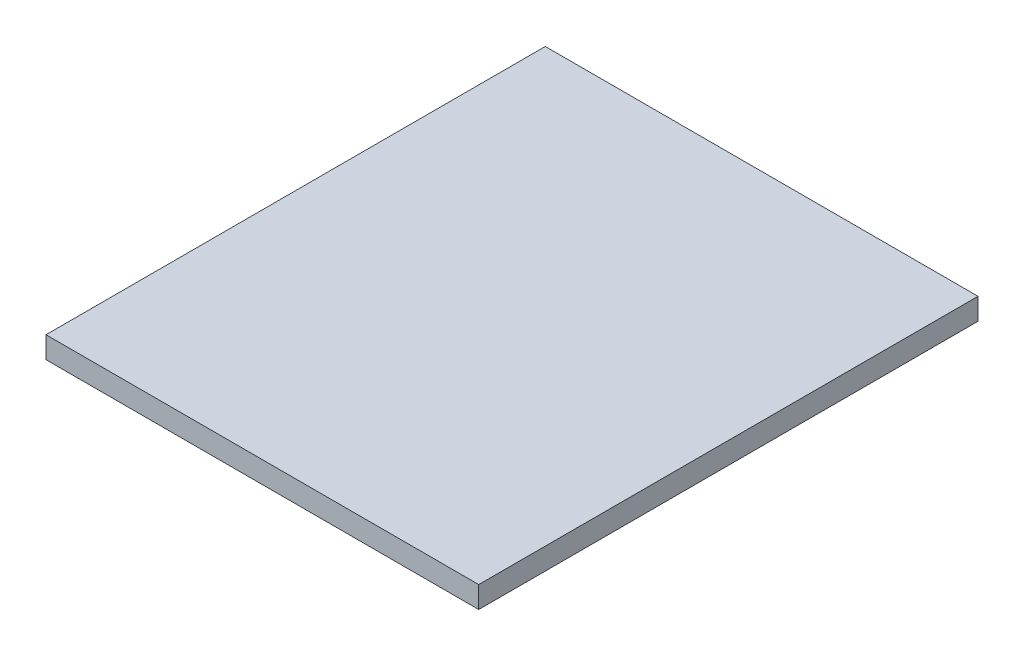
SolidWorks part; units mm, degrees
ref_plane "Front Plane" through (0, 0, 0) normal (0, 0, 1) x (1, 0, 0)
ref_plane "Top Plane" through (0, 0, 0) normal (0, 1, 0) x (1, 0, 0)
ref_plane "Right Plane" through (0, 0, 0) normal (1, 0, 0) x (0, 0, -1)
other "Configuration Table"
sketch "Sketch1" plane through (0, 0, 0) normal (0, 1, 0) x (1, 0, 0)
  line L1 (-65, -75) -> (65, -75)
  line L2 (-65, -75) -> (-65, 75)
  line L3 (-65, 75) -> (65, 75)
  line L4 (65, -75) -> (65, 75)
  line L5 (0, 75) -> (0, -75) construction
  line L6 (-65, 0) -> (65, 0) construction
  point P0 (0, 0)
  dimension "D1" = 130
  dimension "D2" = 150
extrude "Boss-Extrude1" add sketch "Sketch1" along normal blind 6.5
